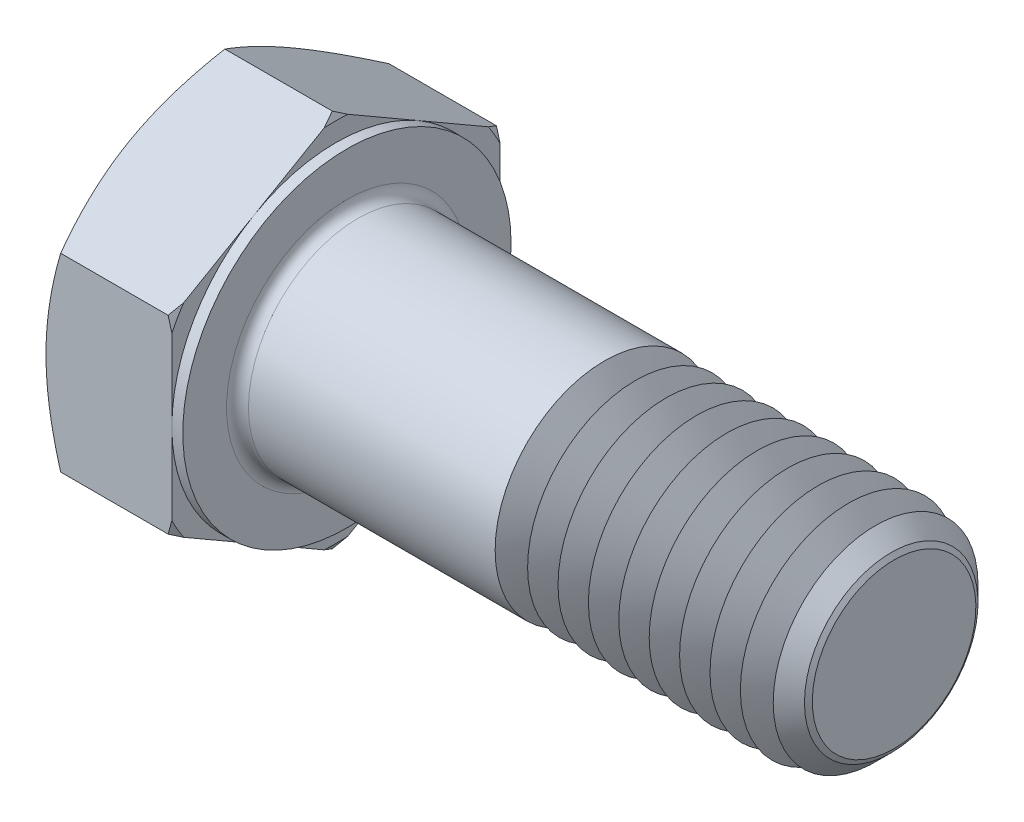
from build123d import *

# Parameters (mm, degrees)
EXTRUDE_364_DEPTH      = 7.5
SKETCH_4_W             = 0.6
SKETCH_4_H             = 11.392304845
CHAMFER_2049_SIZE      = 1.4
FILLET_2094_R          = 0.6
PATTERN_LINEAR_1_COUNT = 10
PATTERN_LINEAR_1_PITCH = 1.666666667


with BuildPart() as part:
    # 草图1 → Extrude 364 (new body)
    with BuildSketch(Plane(origin=(0, 0, 0), x_dir=(0, 0, -1), z_dir=(1, 0, 0))):
        Polygon((9, 5.196152423), (9, -5.196152423), (0, -10.392304845), (-9, -5.196152423), (-9, 5.196152423), (0, 10.392304845), align=None)
    extrude(amount=EXTRUDE_364_DEPTH)

    # 草图2 → 凸台-旋转1 (revolve)
    with BuildSketch(Plane.XY, mode=Mode.PRIVATE) as revolve_1_sk:
        Polygon((0, 0), (37.5, 0), (37.5, 4.4845), (37.5, 6), (7.791693541, 6), (0, 6), align=None)
    revolve(revolve_1_sk.sketch.rotate(Axis((0, 0, 0), (1, 0, 0)), 90), axis=Axis((0, 0, 0), (1, 0, 0)))

    # 草图3 → 切除-旋转1 (revolve, cut)
    with BuildSketch(Plane.XY):
        Polygon((0, 9), (3.690598923, 15.392304845), (3.690598923, 20.392304845), (-10, 20.392304845), (-10, 9), align=None)
    revolve(axis=Axis((0, 0, 0), (1, 0, 0)), mode=Mode.SUBTRACT)

    # 草图5 → 切除-旋转2 (revolve, cut)
    with BuildSketch(Plane.XY):
        Polygon((7.5, 9), (3.809401077, 15.392304845), (3.809401077, 20.392304845), (13.809401077, 20.392304845), (13.809401077, 9), align=None)
    revolve(axis=Axis((0, 0, 0), (1, 0, 0)), mode=Mode.SUBTRACT)

    # 草图4 → 切除-旋转3 (revolve, cut)
    with BuildSketch(Plane.XY, mode=Mode.PRIVATE) as cut_revolve_3_sk:
        with Locations((7.2, 14.696152423)):
            Rectangle(SKETCH_4_W, SKETCH_4_H)
    revolve(cut_revolve_3_sk.sketch.rotate(Axis((0, 0, 0), (1, 0, 0)), 270), axis=Axis((0, 0, 0), (1, 0, 0)), mode=Mode.SUBTRACT)

    # Chamfer 2049
    chamfer_2049_edges = [part.edges().sort_by_distance(p)[0] for p in [
        (37.5, 0, -6),
    ]]
    chamfer(chamfer_2049_edges, length=CHAMFER_2049_SIZE)

    # Fillet 2094
    fillet_2094_edges = [part.edges().sort_by_distance(p)[0] for p in [
        (7.5, 0, -6),
    ]]
    fillet(fillet_2094_edges, radius=FILLET_2094_R)

    # 草图6 → 切除-旋转4 (revolve, cut)
    with BuildSketch(Plane.XY):
        Polygon((22.5, -4.4845), (21.625025667, -6), (21.625025667, -7.5), (23.374974333, -7.5), (23.374974333, -6), align=None)
    cut_revolve_4 = revolve(axis=Axis((-3.175, 0, 0), (1, 0, 0)), mode=Mode.SUBTRACT)

    # 阵列(线性)1: 切除-旋转4 ×10
    with Locations(*[(i * PATTERN_LINEAR_1_PITCH, 0, 0) for i in range(1, PATTERN_LINEAR_1_COUNT)]):
        add(cut_revolve_4, mode=Mode.SUBTRACT)


solid = part.part
